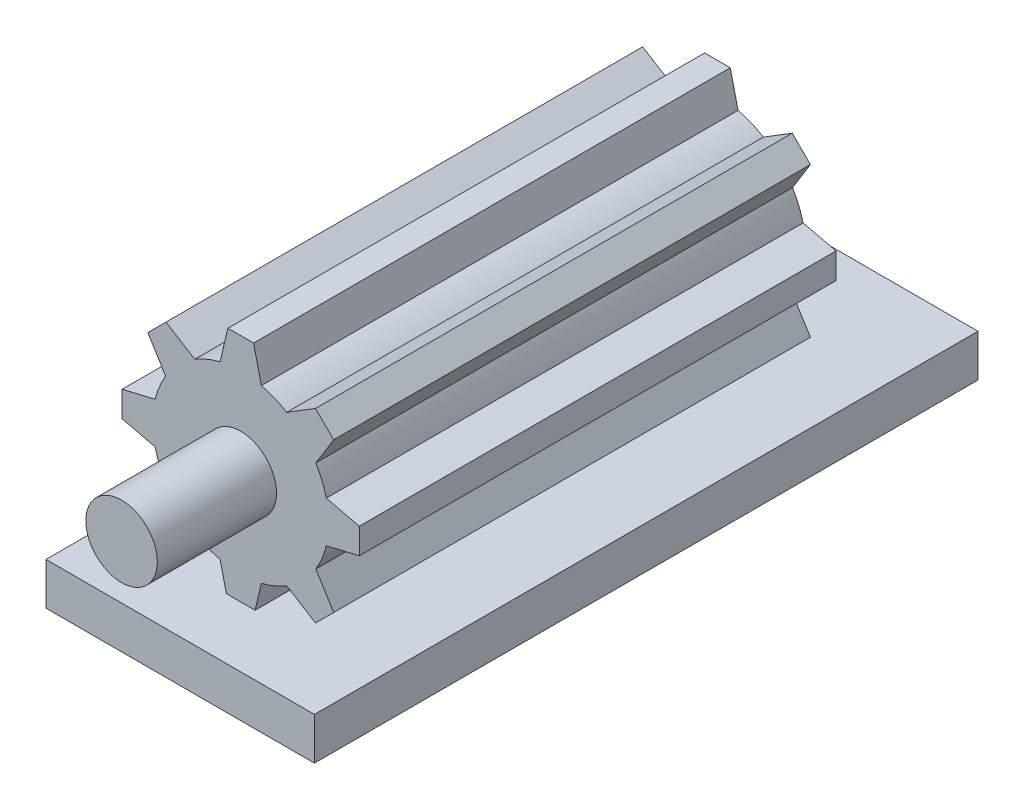
from build123d import *

# Parameters (mm, degrees)
SKETCH1_R                = 150
BOSS_EXTRUDE1_DEPTH      = 3000
CUT_EXTRUDE1_DEPTH       = 435
BOSS_EXTRUDE3_DEPTH      = 2000
BOSS_EXTRUDE4_DEPTH      = 530
BOSS_EXTRUDE4_DEPTH_BACK = 2254
SKETCH5_W                = 1126.0577882
SKETCH5_H                = 177.175277377
BOSS_EXTRUDE5_DEPTH      = 75
SKETCH8_R                = 377.253593713
CUT_EXTRUDE2_DEPTH       = 2500


with BuildPart() as part:
    # Sketch1 → Boss-Extrude1 (new body)
    with BuildSketch(Plane.XY):
        Circle(SKETCH1_R)
    extrude(amount=-BOSS_EXTRUDE1_DEPTH)

    # Sketch2 → Cut-Extrude1 (cut)
    with BuildSketch(Plane(origin=(0, 0, 0), x_dir=(1, 0, 0), z_dir=(0, 1, 0))):
        with BuildLine():
            Line((-50, 150), (-50, 450))
            ThreePointArc((-50, 450), (0, 500), (50, 450))
            Line((50, 450), (50, 150))
            ThreePointArc((50, 150), (0, 100), (-50, 150))
        make_face()
    extrude(amount=CUT_EXTRUDE1_DEPTH, mode=Mode.SUBTRACT)

    # Sketch4 → Boss-Extrude3 (add)
    with BuildSketch(Plane(origin=(0, 0, -3000), x_dir=(-1, 0, 0), z_dir=(0, 0, -1))):
        with BuildLine():
            Line((-86.499256684, 359.11623894), (-53.846539015, 497.477726118))
            Line((-53.846539015, 497.477726118), (53.846539015, 497.477726118))
            Line((53.846539015, 497.477726118), (86.499256684, 359.11623894))
            ThreePointArc((86.499256684, 359.11623894), (141.358201482, 341.268887171), (192.76931682, 315.097738757))
            Line((192.76931682, 315.097738757), (313.694620747, 389.845126508))
            Line((313.694620747, 389.845126508), (389.845126508, 313.694620747))
            Line((389.845126508, 313.694620747), (315.097738757, 192.76931682))
            ThreePointArc((315.097738757, 192.76931682), (341.268887171, 141.358201482), (359.11623894, 86.499256684))
            Line((359.11623894, 86.499256684), (497.477726118, 53.846539015))
            Line((497.477726118, 53.846539015), (497.477726118, -53.846539015))
            Line((497.477726118, -53.846539015), (359.11623894, -86.499256684))
            ThreePointArc((359.11623894, -86.499256684), (341.268887171, -141.358201482), (315.097738757, -192.76931682))
            Line((315.097738757, -192.76931682), (389.845126508, -313.694620747))
            Line((389.845126508, -313.694620747), (313.694620747, -389.845126508))
            Line((313.694620747, -389.845126508), (192.76931682, -315.097738757))
            ThreePointArc((192.76931682, -315.097738757), (141.358201482, -341.268887171), (86.499256684, -359.11623894))
            Line((86.499256684, -359.11623894), (53.846539015, -497.477726118))
            Line((53.846539015, -497.477726118), (-53.846539015, -497.477726118))
            Line((-53.846539015, -497.477726118), (-86.499256684, -359.11623894))
            ThreePointArc((-86.499256684, -359.11623894), (-141.358201482, -341.268887171), (-192.76931682, -315.097738757))
            Line((-192.76931682, -315.097738757), (-313.694620747, -389.845126508))
            Line((-313.694620747, -389.845126508), (-389.845126508, -313.694620747))
            Line((-389.845126508, -313.694620747), (-315.097738757, -192.76931682))
            ThreePointArc((-315.097738757, -192.76931682), (-341.268887171, -141.358201482), (-359.11623894, -86.499256684))
            Line((-359.11623894, -86.499256684), (-497.477726118, -53.846539015))
            Line((-497.477726118, -53.846539015), (-497.477726118, 53.846539015))
            Line((-497.477726118, 53.846539015), (-359.11623894, 86.499256684))
            ThreePointArc((-359.11623894, 86.499256684), (-341.268887171, 141.358201482), (-315.097738757, 192.76931682))
            Line((-315.097738757, 192.76931682), (-389.845126508, 313.694620747))
            Line((-389.845126508, 313.694620747), (-313.694620747, 389.845126508))
            Line((-313.694620747, 389.845126508), (-192.76931682, 315.097738757))
            ThreePointArc((-192.76931682, 315.097738757), (-141.358201482, 341.268887171), (-86.499256684, 359.11623894))
        make_face()
    extrude(amount=BOSS_EXTRUDE3_DEPTH)

    # Sketch5 → Boss-Extrude4 (add, two sides: drawn at the far end of the back side and taken through both)
    with BuildSketch(Plane(origin=(0, 0, -5000), x_dir=(-1, 0, 0), z_dir=(0, 0, -1)).offset(-BOSS_EXTRUDE4_DEPTH_BACK)):
        with Locations((0, -558.816654709)):
            Rectangle(SKETCH5_W, SKETCH5_H)
    extrude(amount=BOSS_EXTRUDE4_DEPTH + BOSS_EXTRUDE4_DEPTH_BACK)

    # Sketch6 → Boss-Extrude5 (add)
    with BuildSketch(Plane(origin=(0, 0, 0), x_dir=(1, 0, 0), z_dir=(0, 1, 0))):
        with BuildLine():
            Line((50, 150), (50, 450))
            ThreePointArc((50, 450), (0, 500), (-50, 450))
            Line((-50, 450), (-50, 150))
            ThreePointArc((-50, 150), (0, 100), (50, 150))
        make_face()
    extrude(amount=BOSS_EXTRUDE5_DEPTH)

    # Sketch8 → Cut-Extrude2 (cut)
    with BuildSketch(Plane.XY):
        Circle(SKETCH8_R)
    extrude(amount=-CUT_EXTRUDE2_DEPTH, mode=Mode.SUBTRACT)


solid = part.part
